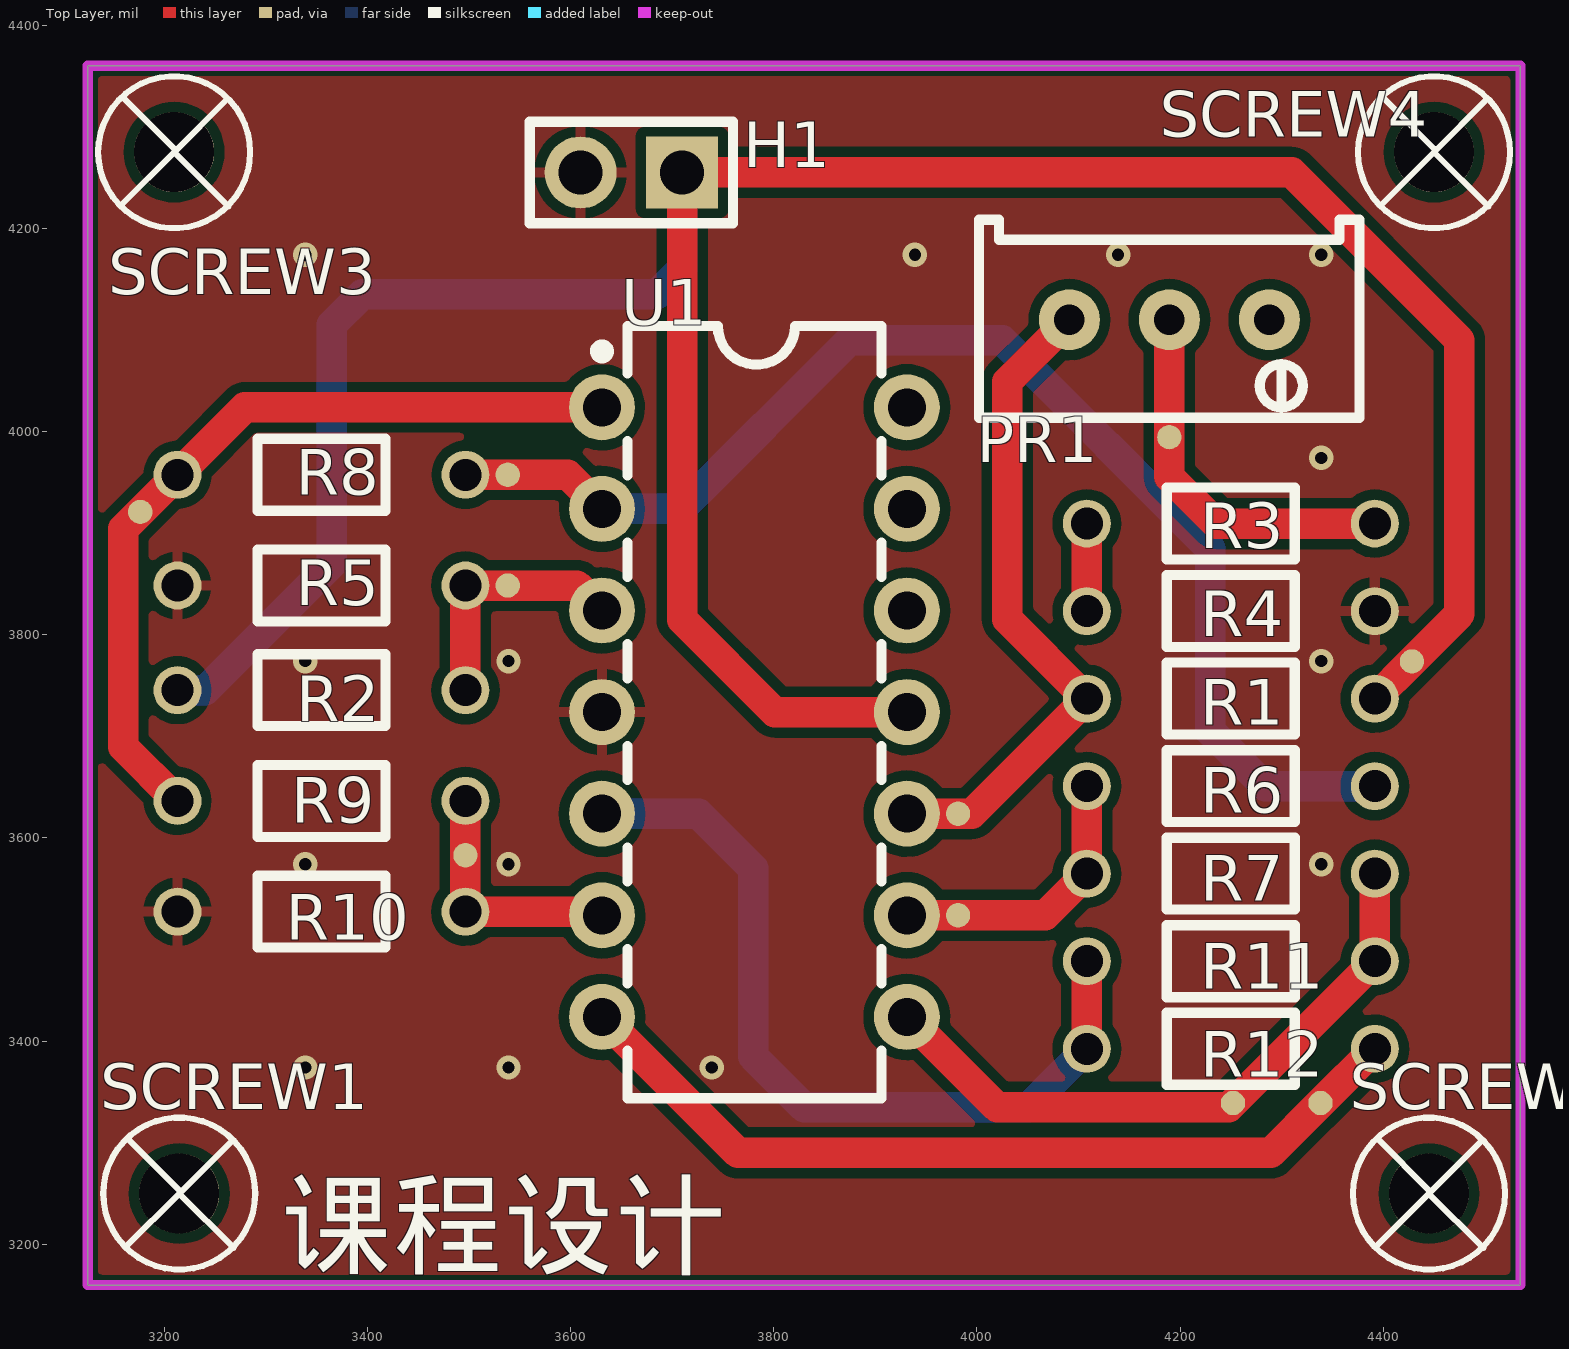
[diagram p0: Top Layer view]
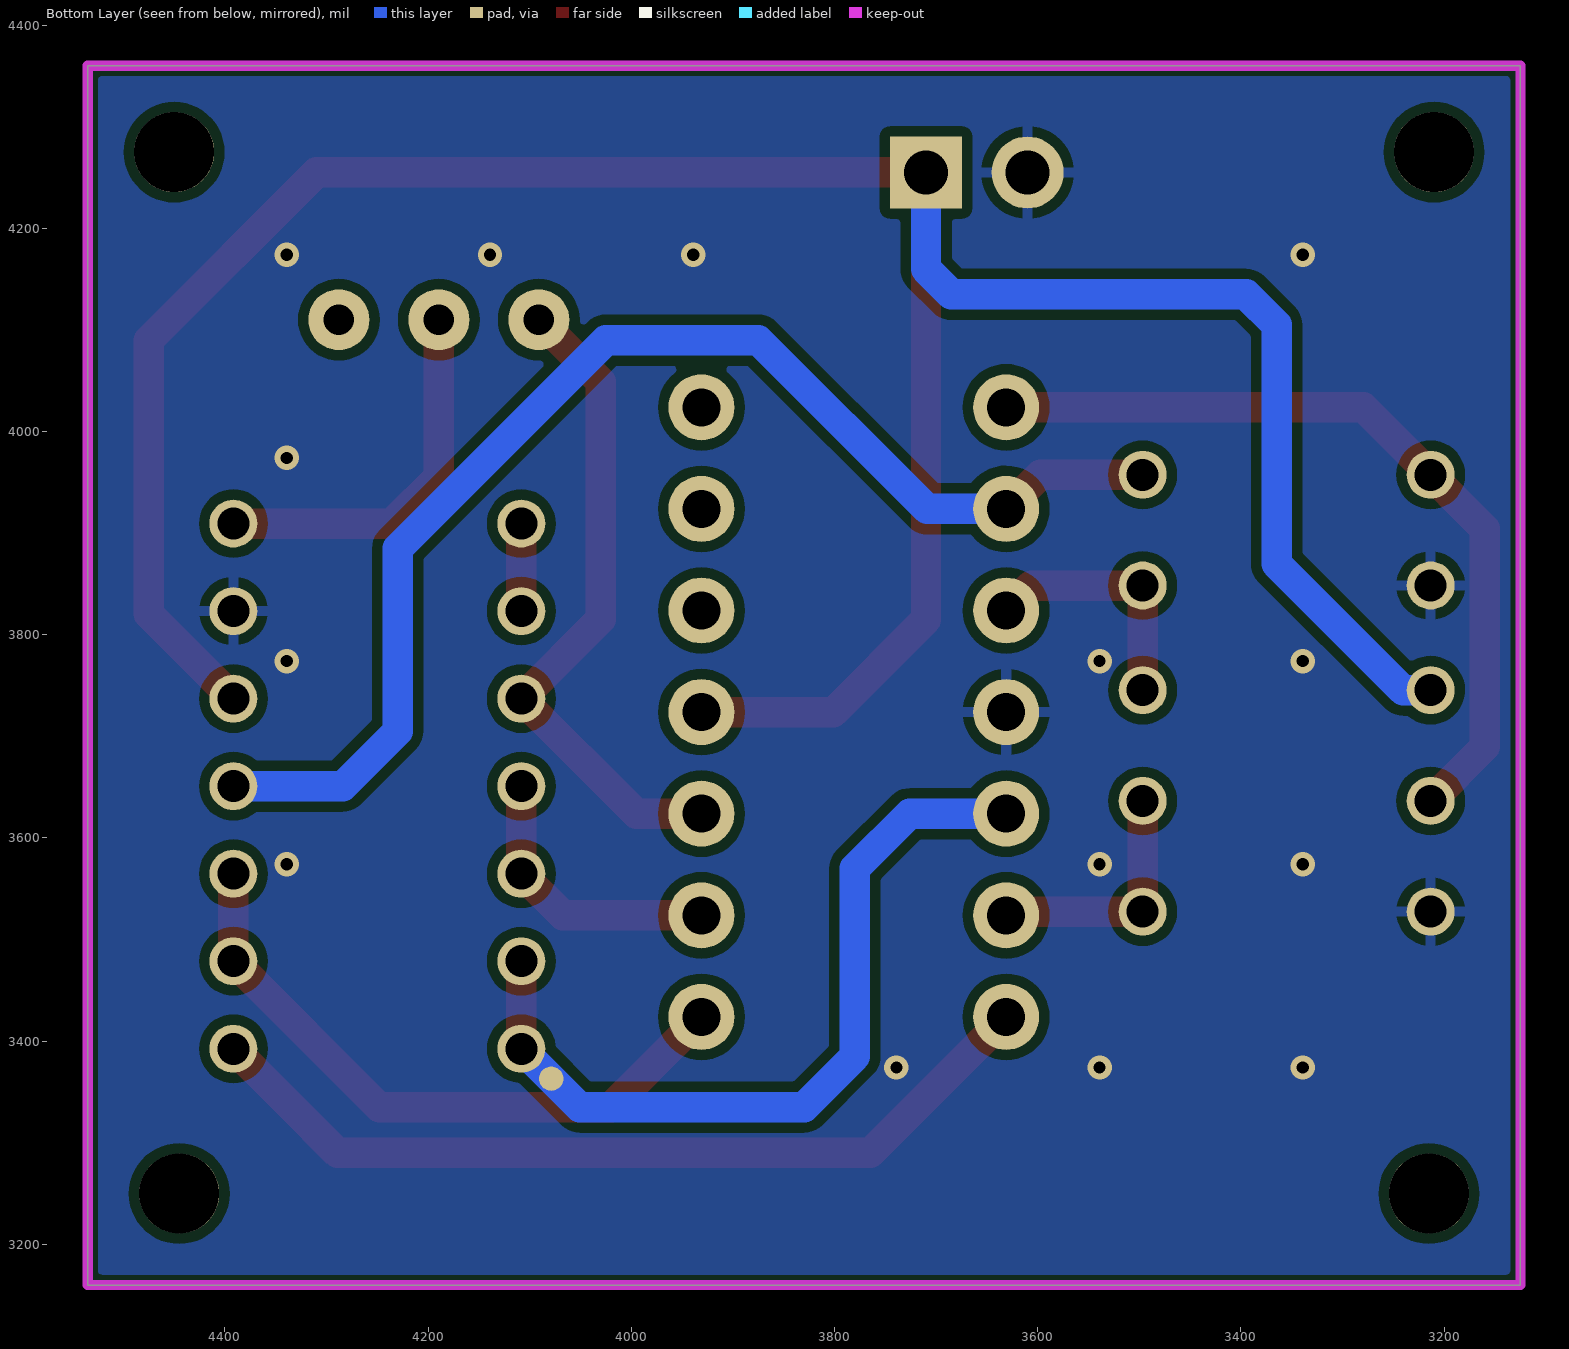
[diagram p1: Bottom Layer view, seen from below]
# Altium PCB MISC51917.pcbdoc
Units mil, origin at the board's own origin, x right, y up, seen from the top; angles counter-clockwise.
Board outline 1410 x 1200 mil, 2 copper layers (Top Layer, Bottom Layer), stack 62.206 mil thick; 19 components, 13 nets, 58 pads, 14 vias.

## Layer stack, top to bottom
Top Solder Mask Layer: solder mask 0.394, Dk 3.3
Top Layer: signal copper 1.379
Dielectric1: surface 59.449, FR4, Dk 4.5
Bottom Layer: signal copper 1.378
Bottom Solder Mask Layer: solder mask 0.394, Dk 3.3

## Board outline
3125,4360 3125,3160 4535,3160 4535,4360

## Design rules (kind name [scope] priority, off if disabled: settings)
BoardOutlineClearance copperThickness2oz_1 [All] p2 off: genericclearance=7.99 ignorepadtopadclearanceinfootprint=FALSE except(0: Arc-SplitContinuation Track-SplitContinuation SMDPad-SplitContinuation THPad-SplitContinuation Via-SplitContinuation Fill-SplitContinuation Region-SplitContinuation Poly-SplitContinuation Text-SplitContinuation Hole-SplitContinuation; 5.98: Arc-CutoutEdge SMDPad-CutoutEdge THPad-CutoutEdge Via-CutoutEdge Fill-CutoutEdge Region-CutoutEdge Text-CutoutEdge; 6.93: Hole-OutlineEdge Hole-CutoutEdge; 10: Poly-OutlineEdge Poly-CutoutEdge; 11.81: Arc-OutlineEdge Track-OutlineEdge SMDPad-OutlineEdge THPad-OutlineEdge Via-OutlineEdge Fill-OutlineEdge Region-OutlineEdge Text-OutlineEdge Track-CutoutEdge)
BoardOutlineClearance copperThickness1oz_1 [All] p4: genericclearance=4.02 ignorepadtopadclearanceinfootprint=FALSE except(0: Arc-SplitContinuation Track-SplitContinuation SMDPad-SplitContinuation THPad-SplitContinuation Via-SplitContinuation Fill-SplitContinuation Region-SplitContinuation Poly-SplitContinuation Text-SplitContinuation Hole-SplitContinuation; 6: SMDPad-CutoutEdge THPad-CutoutEdge Via-CutoutEdge Fill-CutoutEdge Region-CutoutEdge Text-CutoutEdge; 6.93: Hole-OutlineEdge Hole-CutoutEdge; 10: Poly-OutlineEdge Poly-CutoutEdge; 11.8: Arc-OutlineEdge Track-OutlineEdge SMDPad-OutlineEdge THPad-OutlineEdge Via-OutlineEdge Fill-OutlineEdge Region-OutlineEdge Text-OutlineEdge; 11.81: Arc-CutoutEdge Track-CutoutEdge)
Clearance copperThickness2oz [All] p1 off: gap=7.99 ignorepadtopadclearanceinfootprint=FALSE except(5.98: SMDPad-Track SMDPad-SMDPad THPad-Track SMDPad-THPad THPad-THPad Track-Via SMDPad-Via THPad-Via Via-Via Fill-Track Region-Track Fill-SMDPad Region-SMDPad Fill-THPad Region-THPad Fill-Via Region-Via Fill-Fill Fill-Region Region-Region Arc-Track Arc-SMDPad Arc-THPad Arc-Via Fill-Arc Region-Arc Arc-Arc Text-Track SMDPad-Text Text-THPad Text-Via Fill-Text Region-Text Arc-Text Text-Text; 6.93: Hole-Track Hole-SMDPad Hole-THPad Hole-Via Fill-Hole Region-Hole Hole-Arc Hole-Text; 10: Poly-Track Poly-SMDPad Poly-THPad Poly-Via Poly-Fill Poly-Region Poly-Poly Poly-Arc Poly-Text Poly-Hole)
Clearance copperThickness1oz [All] p3: gap=4.02 ignorepadtopadclearanceinfootprint=FALSE except(5.98: SMDPad-Track SMDPad-SMDPad THPad-Track SMDPad-THPad THPad-THPad Track-Via SMDPad-Via THPad-Via Via-Via Fill-Track Region-Track Fill-SMDPad Region-SMDPad Fill-THPad Region-THPad Fill-Via Region-Via Fill-Fill Fill-Region Region-Region; 6: Arc-Track Arc-SMDPad Arc-THPad Arc-Via Fill-Arc Region-Arc Arc-Arc Text-Track SMDPad-Text Text-THPad Text-Via Fill-Text Region-Text Arc-Text Text-Text; 6.93: Hole-Track Hole-SMDPad Hole-THPad Hole-Via Fill-Hole Region-Hole Hole-Arc Hole-Text; 10: Poly-Track Poly-SMDPad Poly-THPad Poly-Via Poly-Fill Poly-Region Poly-Poly Poly-Arc Poly-Text Poly-Hole)
DiffPairsRouting differentialPair [All] p1: maxlimit=6 minlimit=6 mostfreqgap=6 toplayer_minwidth=5 toplayer_prefwidth=10 toplayer_maxwidth=100 toplayer_mingap=6 toplayer_prefgap=6 toplayer_maxgap=6 bottomlayer_minwidth=5 bottomlayer_prefwidth=10 bottomlayer_maxwidth=100 bottomlayer_mingap=6 bottomlayer_prefgap=6 bottomlayer_maxgap=6 maxuncoupledlength=10
HoleToHoleClearance otherClearance [All] p1: gap=11.81 allowstackedmicrovias=TRUE
Length netLength [All] p1: minlimit=0 maxlimit=0
MatchedLengths netLengthTolerance [All] p1: tolerance=1000
PasteMaskExpansion pasteMaskExpansion [All] p1: expansion=0
PlaneConnect innerPlane [All] p1: planeconnectstyle=Relief reliefexpansion=20 reliefentries=4 reliefconductorwidth=10 reliefairgap=10
PolygonConnect copperRegion [(InNet('GND'))] p1: connectstyle=Relief reliefconductorwidth=10 reliefentries=4 polygonreliefangle="90 Angle" airgapwidth=10 via.connectstyle=Relief via.reliefconductorwidth=10 via.reliefentries=4 via.polygonreliefangle="90 Angle" via.airgapwidth=10
RoutingVias viaSize [All] p1: holewidth=12.01 width=24.02 viastyle="Through Hole" minholewidth=11.81 minwidth=19.68 maxholewidth=248.03 maxwidth=393.7
SolderMaskExpansion solderMaskExpansion [IsVia] p1: expansion=-1000 istentingtop=TRUE
SolderMaskExpansion solderMaskExpansion [All] p2: expansion=2 istentingtop=FALSE
Width copperThickness2oz_2 [All] p1 off: maxlimit=100 minlimit=8 preferedwidth=10
Width copperThickness1oz_2 [All] p2: maxlimit=100 minlimit=5 preferedwidth=10

## Components (designator, comment, footprint, x,y, rotation, side; value= is the part's Value field where it differs from the comment)
H1 "" HDR-TH_2P-P2.54-V-M-1 3660,4255 r180 top
PR1 "10kΩ" R_3296 4189.5,4105.07 r180 top
R1 "10kΩ" Res_1/8W 4250,3734.66 r0 top
R2 "10kΩ" Res_1/8W 3355,3747.95 r180 top
R3 "9.76kΩ" Res_1/8W 4250,3906.97 r0 top
R4 "140Ω" Res_1/8W 4250,3825.77 r180 top
R5 "10kΩ" Res_1/8W 3355,3846 r0 top
R6 "2.2kΩ" Res_1/8W 4250,3648.51 r0 top
R7 "10kΩ" Res_1/8W 4250,3567.31 r180 top
R8 "10kΩ" Res_1/8W 3355,3955 r0 top
R9 "10kΩ" Res_1/8W 3355,3638.95 r180 top
R10 "100kΩ" Res_1/8W 3355,3525 r0 top
R11 "10kΩ" Res_1/8W 4250,3476.2 r0 top
R12 "100kΩ" Res_1/8W 4250,3395 r180 top
SCREW1 "" M2螺丝 3215,3250 r0 top
SCREW2 "" M2螺丝 4445,3250 r0 top
SCREW3 "" M2螺丝 3210,4275 r0 top
SCREW4 "" M2螺丝 4450,4275 r0 top
U1 "LM324N/PB" PDIP-14_L19.2-W6.6-P2.54-LS7.6-BL 3781.07,3723.88 r270 top

## Footprints (in the part's own frame and the unit in brackets; to place one, negate y for a bottom-side part, rotate by r counter-clockwise, add the part's x,y. Pads: shape width x height; smd on the part's side, far side on the other; paste and mask are expansions set on the pad)
HDR-TH_2P-P2.54-V-M-1 [mm]
  rect 1.8x1.8 hole 1.1: 1(-1.27,0)
  round 1.8 hole 1.1: 2(1.27,0)
  silkscreen extent -2.54,-1.27 2.54,1.27
M2螺丝 [mm]
  round 2 hole 2: 1(0,0)
  silkscreen extent -1.9,-1.9 1.9,1.9
PDIP-14_L19.2-W6.6-P2.54-LS7.6-BL [mm]
  round 1.65 hole 0.95: 1(-7.62,-3.81) 2(-5.08,-3.81) 3(-2.54,-3.81) 4(0,-3.81) 5(2.54,-3.81) 6(5.08,-3.81) 7(7.62,-3.81) 8(7.62,3.81) 9(5.08,3.81) 10(2.54,3.81) 11(0,3.81) 12(-2.54,3.81) 13(-5.08,3.81) 14(-7.62,3.81)
  silkscreen extent -9.65,-3.96 9.65,3.17
R_3296 [mil]
  round 60 hole 30 paste+0 mask+2: 1(-98.4,-5) 2(0,-5) 3(98.4,-5)
  silkscreen extent -187,-103 187,91
Res_1/8W [mil]
  round 47.2 hole 31.5 paste+0 mask+2: 1(-141.7,2.48) 2(141.7,2.48)
  silkscreen extent -63,-33 63,38

## Free pads (board coordinates)
  round 24 smd: TP1(4189.5,3994.57) TP2(3981.54,3623.88) TP3(4428.3,3773.74) TP4(3538.28,3848.48) TP5(3981.54,3523.88) TP6(3538.28,3957.48) TP7(4252.15,3339.12) TP8(3176.7,3920.88) TP9(3496.7,3583.08) TP11(4338.3,3339.12)
  round 24 smd far side: TP10(4078.9,3363.12)

## Via types
v1: diameter 24.02, hole 12, Top Layer to Bottom Layer, 14 vias

## Nets (pads, with @x,y where several pads share a name; then routed paths per layer and width w, separated by ;. In a path a pad name is that pad's centre, name@x,y a point inside that pad or via, vN(x,y) a via of type N, cw(c..) or ccw(c..) an arc to the next point about the centre after c; other vN are vias at no path point)
10V: H1.1 pad.TP3 R1.2 R2.2 U1.11 | length 2821.3
  Top Layer w30: U1.11 3801.12,3723.88 3710,3815 H1.1 4310,4255 4475,4090 4475,3820.44 pad.TP3 R1.2
  Bottom Layer w30: R2.2 3240.48,3745.48 3365,3870 3365,4105 3395,4135 3685,4135 3710,4160 H1.1@3710,4255.7
$1N2: pad.TP1 PR1.2 R3.2 | length 375.8
  Top Layer w30: PR1.2 pad.TP1 4189.5,3955.5 4235.55,3909.45 R3.2
$1N3: pad.TP2 PR1.3 R1.1 U1.10 | length 654.8
  Top Layer w30: U1.10 3995.04,3623.88 R1.1 4030,3815.44 4030,4048.97 PR1.3
$1N4: R3.1 R4.2 | length 86.2
  Top Layer w30: R4.2 R3.1
$1N6: pad.TP4 R2.1 R5.2 U1.3 | length 247.6
  Top Layer w30: R2.1 R5.2 3606.48,3848.48 U1.3
$1N7: pad.TP6 R6.2 R8.2 U1.2 | length 1265
  Top Layer w30: R8.2 3597.48,3957.48 U1.2
  Bottom Layer w30: U1.2 3708.88,3923.88 3875,4090 4025,4090 4230,3885 4230,3705 4284.02,3650.99 R6.2
$1N8: pad.TP5 R6.1 R7.2 U1.9 | length 280.3
  Top Layer w30: U1.9 4067.35,3523.88 R7.2 R6.1
$1N9: pad.TP8 R8.1 R9.2 U1.1 | length 810.4
  Top Layer w30: R9.2 3160,3689.78 3160,3904.18 pad.TP8 R8.1 3279.7,4023.88 U1.1
$1N12: pad.TP9 R9.1 R10.2 U1.6 | length 244.9
  Top Layer w30: R9.1 pad.TP9 R10.2 3627.48,3527.48 U1.6
$1N16: pad.TP10 R11.1 R12.2 U1.5 | length 815.2
  Top Layer w30: R12.2 R11.1
  Bottom Layer w30: U1.5 3726.12,3623.88 3780,3570 3780,3385 3830,3335 4050.78,3335 R12.2
$1N17: pad.TP7 R7.1 R11.2 U1.8 | length 643.1
  Top Layer w30: U1.8 4019.95,3335 4248.02,3335 R11.2 R7.1
$1N18: pad.TP11 R12.1 U1.7 | length 858.5
  Top Layer w30: U1.7 3764.95,3290 4289.18,3290 pad.TP11 R12.1
GND: H1.2 R4.1 R5.1 R10.1 U1.4
  other v1: 3339.1,3374.1 3539.1,3374.1 3739.1,3374.1 3339.1,3574.1 3539.1,3574.1 4339.1,3574.1 3339.1,3774.1 3539.1,3774.1 4339.1,3774.1 4339.1,3974.1 3339.1,4174.1 3939.1,4174.1 4139.1,4174.1 4339.1,4174.1
pads on no net: PR1.1 SCREW1.1 SCREW2.1 SCREW3.1 SCREW4.1 U1.12 U1.13 U1.14

## Polygon pours and split planes (outlines as drawn)
GND on Top Layer (solid, remove dead copper, pour order 0): 3000,4505 3000,3000 4725,3000 4725,4505
GND on Bottom Layer (solid, remove dead copper, pour order 2): 3045,4485 3045,3025 4800,3025 4800,4485

## Keep-outs
Board Outline Layer:
  the board outline again, w10

## Silkscreen, mask and mechanical layers (free items; w line width, h text height)
Top Silkscreen Layer:
  text "课程设计" at 3315,3180 h80